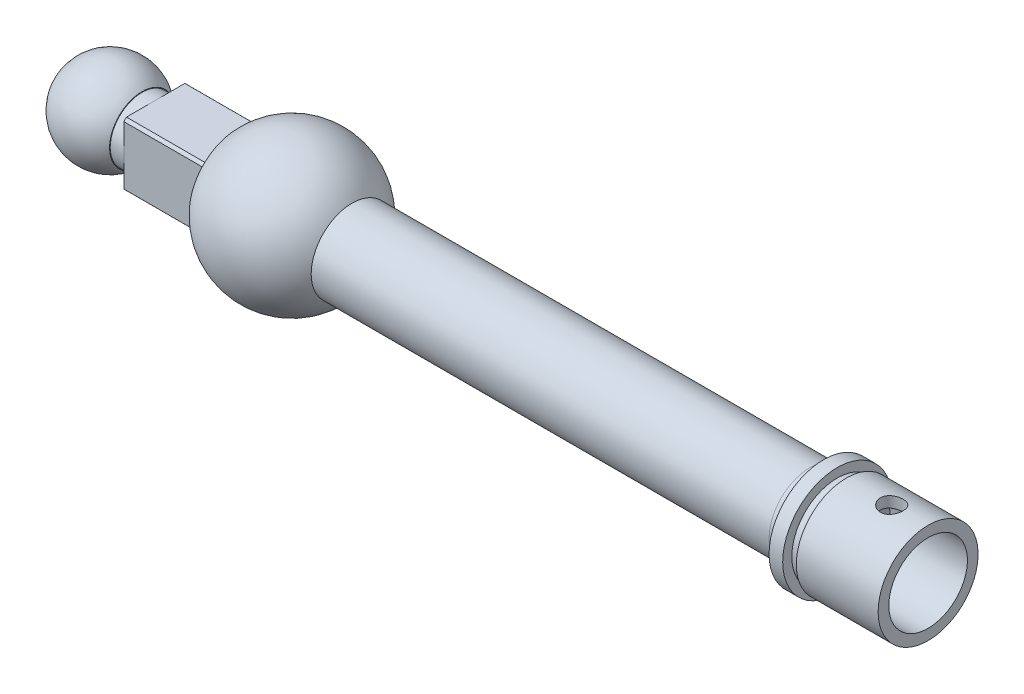
from build123d import *

# Parameters (mm, degrees)
SKETCH2_R          = 25.69251773
SKETCH2_W          = 14
SKETCH2_H          = 14
CUT_EXTRUDE1_DEPTH = 18
SKETCH4_R          = 2.5
CUT_EXTRUDE3_DEPTH = 10


with BuildPart() as part:
    # Sketch1 → Revolve1 (revolve)
    with BuildSketch(Plane.XY, mode=Mode.PRIVATE) as revolve1_sk:
        with BuildLine():
            Line((254.379291769, 33.201574447), (254.379291769, 30.851574447))
            Line((254.379291769, 30.851574447), (237.379291769, 30.851574447))
            Line((237.379291769, 30.851574447), (234.379291769, 26.201574447))
            Line((234.379291769, 26.201574447), (172.647910202, 26.201574447))
            Line((172.647910202, 26.201574447), (66.379291769, 26.201574447))
            Line((66.379291769, 26.201574447), (66.379291769, 28.201574447))
            ThreePointArc((66.379291769, 28.201574447), (73.620533102, 32.172747161), (81.379291769, 29.343002876))
            Line((81.379291769, 29.343002876), (81.379291769, 29.201574447))
            Line((81.379291769, 29.201574447), (84.379291769, 29.201574447))
            Line((84.379291769, 29.201574447), (84.379291769, 31.701574447))
            Line((84.379291769, 31.701574447), (102.379291769, 31.701574447))
            Line((102.379291769, 31.701574447), (102.379291769, 32.784579692))
            ThreePointArc((102.379291769, 32.784579692), (115.381258369, 38.170170595), (127.608048324, 31.201574447))
            Line((127.608048324, 31.201574447), (228.379291769, 31.201574447))
            ThreePointArc((228.379291769, 31.201574447), (230.500612112, 32.080254104), (231.379291769, 34.201574447))
            Line((231.379291769, 34.201574447), (234.379291769, 34.201574447))
            Line((234.379291769, 34.201574447), (234.379291769, 32.201574447))
            Line((234.379291769, 32.201574447), (236.379291769, 32.201574447))
            Line((236.379291769, 32.201574447), (236.379291769, 33.201574447))
            Line((236.379291769, 33.201574447), (254.379291769, 33.201574447))
        make_face()
    revolve(revolve1_sk.sketch.rotate(Axis((62.379291769, 22.201574447, 0), (1, 0, 0)), 90), axis=Axis((62.379291769, 22.201574447, 0), (1, 0, 0)))

    # Sketch2 → Cut-Extrude1 (cut)
    with BuildSketch(Plane.ZY.offset(-84.379291769)):
        with Locations((0, 22.201574447)):
            Circle(SKETCH2_R)
        with Locations((0, 22.201574447)):
            Rectangle(SKETCH2_W, SKETCH2_H, mode=Mode.SUBTRACT)
    extrude(amount=-CUT_EXTRUDE1_DEPTH, mode=Mode.SUBTRACT)

    # Sketch4 → Cut-Extrude3 (cut)
    with BuildSketch(Plane(origin=(0, 29.201574447, 0), x_dir=(1, 0, 0), z_dir=(0, 1, 0))):
        with Locations(Location((246.379291769, 0, 0), (0, 0, 90))):
            Circle(SKETCH4_R)
    extrude(amount=CUT_EXTRUDE3_DEPTH, mode=Mode.SUBTRACT)


solid = part.part
